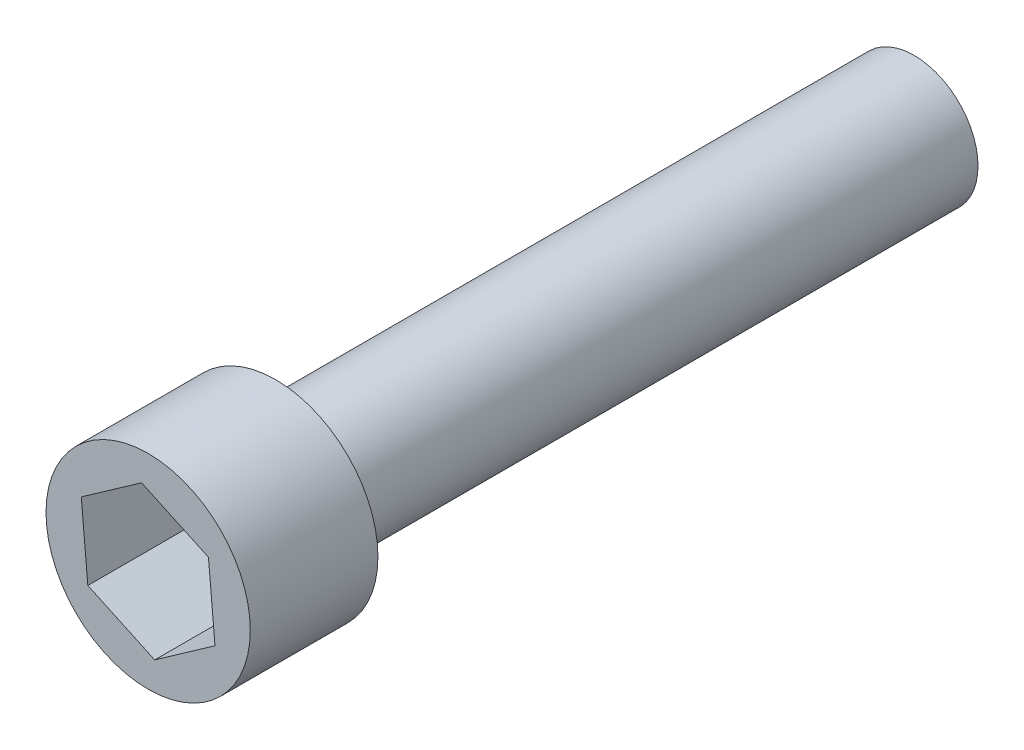
from build123d import *

# Parameters (mm, degrees)
SKETCH1_R           = 5
BOSS_EXTRUDE1_DEPTH = 50
SKETCH2_R           = 8
BOSS_EXTRUDE2_DEPTH = 10
CUT_EXTRUDE1_DEPTH  = 8


with BuildPart() as part:
    # Sketch1 → Boss-Extrude1 (new body)
    with BuildSketch(Plane.XY):
        Circle(SKETCH1_R)
    extrude(amount=BOSS_EXTRUDE1_DEPTH)

    # Sketch2 → Boss-Extrude2 (add)
    with BuildSketch(Plane.XY.offset(50)):
        Circle(SKETCH2_R)
    extrude(amount=BOSS_EXTRUDE2_DEPTH)

    # Sketch3 → Cut-Extrude1 (cut)
    with BuildSketch(Plane.XY.offset(60)):
        Polygon((0.514138009, -5.750564793), (5.237204202, -2.430025819), (4.723066192, 3.320538974), (-0.514138009, 5.750564793), (-5.237204202, 2.430025819), (-4.723066192, -3.320538974), align=None)
    extrude(amount=-CUT_EXTRUDE1_DEPTH, mode=Mode.SUBTRACT)


solid = part.part
